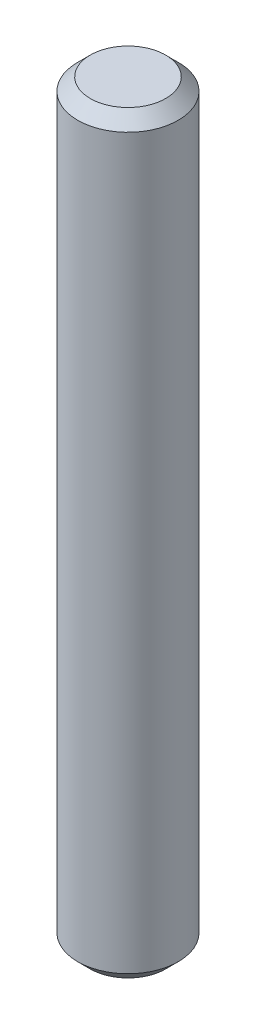
from build123d import *

# Parameters (mm, degrees)
SKETCH1_R           = 2
BOSS_EXTRUDE1_DEPTH = 30
CHAMFER1_SIZE       = 0.5


with BuildPart() as part:
    # Sketch1 → Boss-Extrude1 (new body)
    with BuildSketch(Plane(origin=(0, 0, 0), x_dir=(1, 0, 0), z_dir=(0, 1, 0))):
        with Locations(Location((0, 0, 0), (0, 0, 270))):
            Circle(SKETCH1_R)
    extrude(amount=-BOSS_EXTRUDE1_DEPTH)

    # Chamfer1
    chamfer1_edges = [part.edges().sort_by_distance(p)[0] for p in [
        (0, 0, -2),
        (0, -30, -2),
    ]]
    chamfer(chamfer1_edges, length=CHAMFER1_SIZE)


solid = part.part
